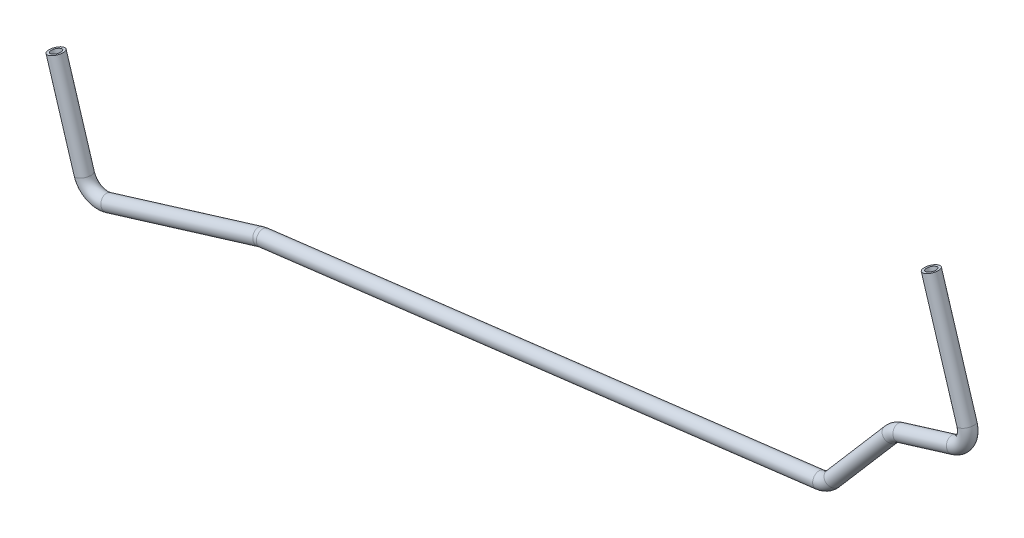
from build123d import *

# Parameters (mm, degrees)
SWEEP_THIN1_PROFILE_R   = 15
SWEEP_THIN1_PROFILE_R_2 = 10


with BuildPart() as part:
    # Sweep-Thin1: sweep along a curve in space
    with BuildLine() as sweep_thin1_path:
        Line((2022.793428066, 28.838151427, -11.649730724), (1949.498015394, 268.099387204, -11.649730724))
        ThreePointArc((1996.263961553, -21.123708091, -11.649730724), (2019.876134716, -1.637210748, -11.649730724), (2022.793428066, 28.838151427, -11.649730724))
        Line((1886.137822525, -54.859807379, -11.649730724), (1996.263961553, -21.123708091, -11.649730724))
        ThreePointArc((1867.261044608, -67.278310178, -10.899623065), (1875.803940416, -59.718953476, -11.458302347), (1886.137822525, -54.859807379, -11.649730724))
        Line((1758.437618296, -195.5154797, -0.172125022), (1867.261044608, -67.278310178, -10.899623065))
        ThreePointArc((1732.773486814, -209.353915035, 0.825071817), (1746.915200671, -204.846187229, 0.566882239), (1758.437618296, -195.5154797, -0.172125022))
        Line((587.398241077, -350.636667449, 0.825071817), (1732.773486814, -209.353915035, 0.825071817))
        ThreePointArc((580.57895604, -352.090126062, 0.825071817), (583.956868872, -351.214528548, 0.825071817), (587.398241077, -350.636667449, 0.825071817))
        Line((580.57895604, -352.090126062, 0.825071817), (267.840903589, -447.894465358, 0.825071817))
        ThreePointArc((267.840903589, -447.894465358, 0.825071817), (237.365541414, -444.977172008, 0.825071817), (217.879044071, -421.364998844, 0.825071817))
        Line((217.879044071, -421.364998844, 0.825071817), (159.847616861, -231.930619776, 0.825071817))
    # Sweep-Thin1 profile (on start of the path) → Sweep-Thin1 (sweep)
    with BuildSketch(Plane(origin=(159.847616861, -231.930619776, 0.825071817), x_dir=(-0.9561415753975281, -0.2929049125507002, 0), z_dir=(0.2929049125507002, -0.9561415753975281, -2.7998246546986226e-14))):
        Circle(SWEEP_THIN1_PROFILE_R)
        Circle(SWEEP_THIN1_PROFILE_R_2, mode=Mode.SUBTRACT)
    sweep(path=sweep_thin1_path.line)


solid = part.part
